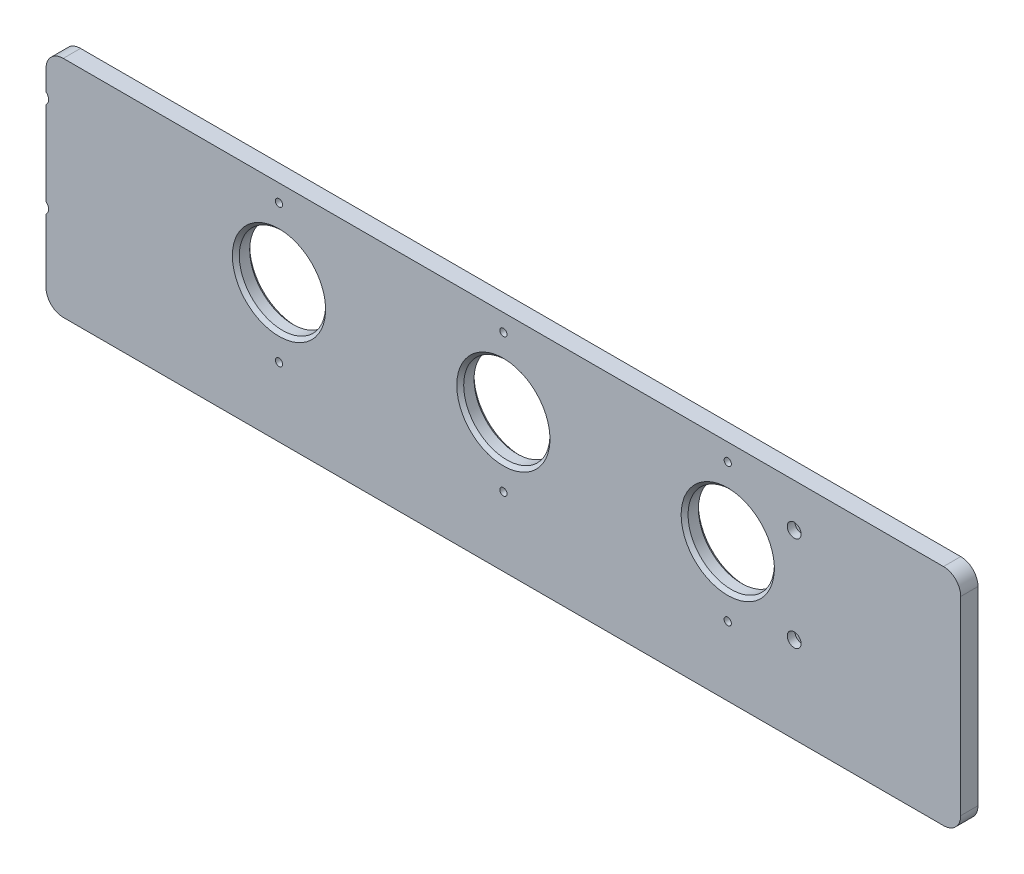
SolidWorks part; units mm, degrees
material "A6061"
ref_plane "前视" through (0, 0, 0) normal (0, 0, 1) x (1, 0, 0)
ref_plane "上视" through (0, 0, 0) normal (0, 1, 0) x (1, 0, 0)
ref_plane "右视" through (0, 0, 0) normal (1, 0, 0) x (0, 0, -1)
sketch "草图1" plane through (0, 0, 0) normal (0, 0, 1) x (1, 0, 0)
  line L1 (-265, -65) -> (265, -65)
  line L2 (-265, -65) -> (-265, 65)
  line L3 (-265, 65) -> (265, 65)
  line L4 (265, -65) -> (265, 65)
  line L5 (-265, -65) -> (265, 65) construction
  line L6 (-265, 65) -> (265, -65) construction
  point P0 (0, 0)
  dimension "D1" = 530
  dimension "D2" = 130
extrude "凸台-拉伸1" add sketch "草图1" along normal blind 10
hole_wizard "M4 六角凹头螺钉的柱形沉头孔1" positions "草图8" profile "草图9" counterbore size "M4" standard "ISO" end condition through all
sketch "草图8" plane through (0, 0, 10) normal (0, 0, -1) x (-1, 0, 0)
  line L0 (-265, -65) -> (-265, 65) construction
  line L1 (265, -65) -> (-265, -65) construction
  point P0 (-168.5, -15)
  point P2 (-168.5, 40)
  dimension "D1" = 96.5
  dimension "D2" = 50
  dimension "D3" = 55
sketch "草图9" plane through (168.5, -15, 10) normal (1, 0, 0) x (0, -1, 0)
  line L0 (0, 0) -> (0, 10)
  line L1 (0, 10) -> (2.25, 10)
  line L3 (2.25, 10) -> (2.25, 4.4)
  line L4 (2.25, 4.4) -> (4, 4.4)
  line L5 (4, 4.4) -> (4, 0)
  line L7 (4, 0) -> (0, 0)
  line L11 (0, -6.35) -> (0, 107.95) construction
  dimension "通孔孔直径" = 4.5
  dimension "通孔孔深度" = 10
  dimension "柱形沉头孔直径" = 8
  dimension "柱形沉头孔深度" = 4.4
pattern_linear "阵列(线性)1" count 2 spacing 436 along (-1, 0, 0) of "M4 六角凹头螺钉的柱形沉头孔1"
sketch "草图14" plane through (0, 0, 10) normal (0, 0, 1) x (1, 0, 0)
  line L0 (265, 65) -> (-265, 65) construction
  circle A0 centre (-130, 15) radius 25
  circle A1 centre (0, 15) radius 25
  circle A2 centre (130, 15) radius 25
  dimension "D1" = 50
  dimension "D2" = 50
  dimension "D5" = 130
  dimension "D6" = 130
  dimension "D3" = 0
  dimension "D4" = 0
  dimension "D7" = 0
extrude "切除-拉伸1" cut sketch "草图14" against normal through all
chamfer "倒角1" distance 2 angle 45 6 edges at (155, 15, 10) (155, 15, 0) (25, 15, 10) (25, 15, 0) (-105, 15, 10) (-105, 15, 0)
hole_wizard "M5 螺纹孔2" positions "草图15" profile "草图16" tap size "M5" standard "ISO" end condition through all
sketch "草图15" plane through (0, 0, 10) normal (0, 0, 1) x (1, 0, 0)
  circle A0 centre (-130, 15) radius 40
  circle A1 centre (0, 15) radius 40
  circle A2 centre (130, 15) radius 40
  point P11 (-130, -25)
  point P13 (-130, 55)
  point P15 (0, 55)
  point P17 (0, -25)
  point P19 (130, -25)
  point P21 (130, 55)
  dimension "D1" = 80
sketch "草图16" plane through (130, 55, 10) normal (1, 0, 0) x (0, -1, 0)
  line L0 (0, 0) -> (0, 10)
  line L1 (0, 10) -> (2.1, 10)
  line L2 (2.1, 10) -> (2.1, 0)
  line L5 (2.1, 0) -> (0, 0)
  line L11 (0, -6.35) -> (0, 107.95) construction
  dimension "通孔螺纹孔钻头直径" = 4.2
  dimension "通孔螺纹孔钻头深度" = 10
cosmetic thread "孔螺蚊线10" parameters "D2"=5
cosmetic thread "孔螺蚊线11" parameters "D2"=5
cosmetic thread "孔螺蚊线12" parameters "D2"=5
cosmetic thread "孔螺蚊线13" parameters "D2"=5
cosmetic thread "孔螺蚊线14" parameters "D2"=5
cosmetic thread "孔螺蚊线15" parameters "D2"=5
fillet "圆角1" radius 10 4 edges at (-265, 65, 5) (-265, -65, 5) (265, 65, 5) (265, -65, 5)
